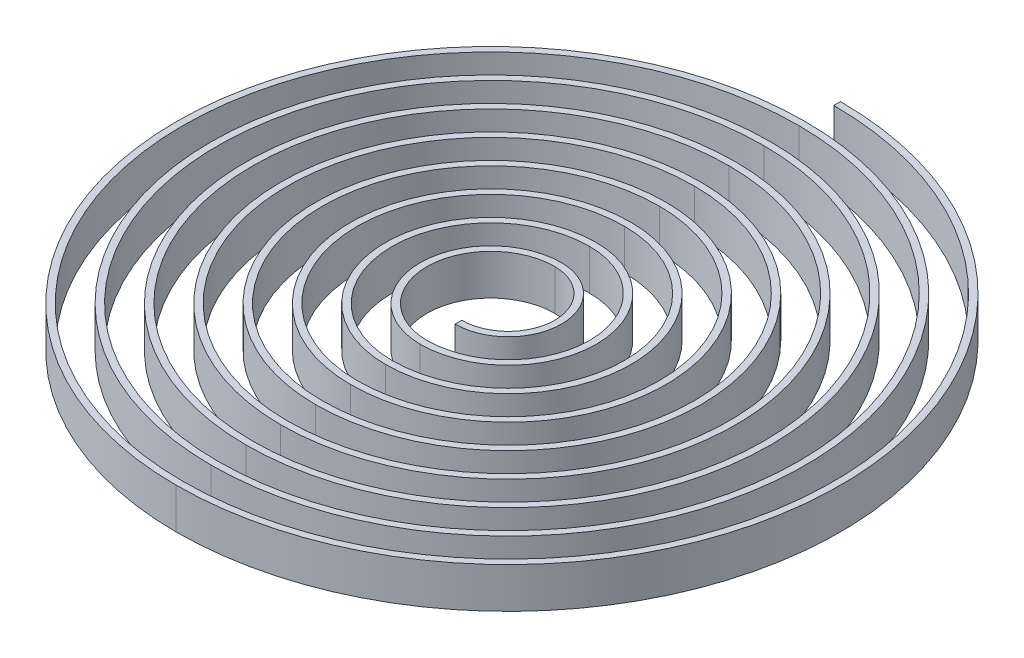
SolidWorks part; units mm, degrees
ref_plane "Front plane" through (0, 0, 0) normal (0, 0, 1) x (1, 0, 0)
ref_plane "Top plane" through (0, 0, 0) normal (0, 1, 0) x (1, 0, 0)
ref_plane "Right plane" through (0, 0, 0) normal (1, 0, 0) x (0, 0, -1)
other "Configuration Table"
sketch "Sketch 1" plane through (0, 0, 0) normal (0, 1, 0) x (1, 0, 0)
  arc A0 (0, -2.5) -> (0, 2.5) centre (0, 0) ccw
  arc A1 (0, 2.5) -> (0, -4.375) centre (0, -0.9375) ccw
  arc A2 (0, -4.375) -> (0, 4.375) centre (0, 0) ccw
  arc A3 (0, 4.375) -> (0, -6.25) centre (0, -0.9375) ccw
  arc A4 (0, -6.25) -> (0, 6.25) centre (0, 0) ccw
  arc A5 (0, 6.25) -> (0, -8.125) centre (0, -0.9375) ccw
  arc A6 (0, -8.125) -> (0, 8.125) centre (0, 0) ccw
  arc A7 (0, 8.125) -> (0, -10) centre (0, -0.9375) ccw
  arc A8 (0, -10) -> (0, 10) centre (0, 0) ccw
  arc A9 (0, 10) -> (0, -11.875) centre (0, -0.9375) ccw
  arc A10 (0, -11.875) -> (0, 11.875) centre (0, 0) ccw
  arc A11 (0, 11.875) -> (0, -13.75) centre (0, -0.9375) ccw
  arc A12 (0, -13.75) -> (0, 13.75) centre (0, 0) ccw
  arc A13 (0, 13.75) -> (0, -15.625) centre (0, -0.9375) ccw
  arc A14 (0, -15.625) -> (0, 15.625) centre (0, 0) ccw
  arc A15 (0, 15.625) -> (0, -17.5) centre (0, -0.9375) ccw
  arc A16 (0, -17.5) -> (0, 17.5) centre (0, 0) ccw
extrude "Extrude-thin 2" add sketch "Sketch 1" along normal blind 2.18 thin
